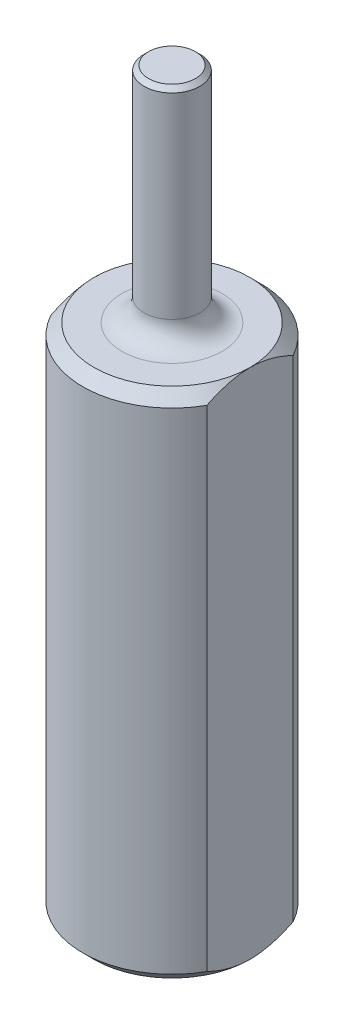
from build123d import *

# Parameters (mm, degrees)
HOLE_WIZARD_M3_1_D     = 2.5
HOLE_WIZARD_M3_1_DEPTH = 11.5
HOLE_WIZARD_M3_1_TIP   = 0.751075774
CHAMFER_1_SIZE         = 0.5
FILLET_1_R             = 1
SKETCH_4_W             = 0.5
SKETCH_4_H             = 23
CUT_EXTRUDE_1_DEPTH    = 5
CHAMFER_2_SIZE         = 0.2


with BuildPart() as part:
    # 草图1 → 旋转1 (revolve)
    with BuildSketch(Plane.XY, mode=Mode.PRIVATE) as revolve_1_sk:
        Polygon((1.25, 33), (1.25, 23), (4, 23), (4, 0), (0, 0), (0, 33), align=None)
    revolve(revolve_1_sk.sketch.rotate(Axis((0, -0.524377328, 0), (0, 1, 0)), 90), axis=Axis((0, -0.524377328, 0), (0, 1, 0)))

    # M3 螺纹孔1
    with Locations(Plane(origin=(0, 0, 0), x_dir=(-1, 0, 0), z_dir=(0, -1, 0))):
        with Locations((0, 0)):
            Hole(HOLE_WIZARD_M3_1_D / 2, depth=HOLE_WIZARD_M3_1_DEPTH)
            with Locations((0, 0, -(HOLE_WIZARD_M3_1_DEPTH + HOLE_WIZARD_M3_1_TIP / 2))):  # 118° drill point
                Cone(0, HOLE_WIZARD_M3_1_D / 2, HOLE_WIZARD_M3_1_TIP, mode=Mode.SUBTRACT)

    # 倒角1
    chamfer_1_edges = [part.edges().sort_by_distance(p)[0] for p in [
        (0, 0, 4),
        (0, 23, 4),
    ]]
    chamfer(chamfer_1_edges, length=CHAMFER_1_SIZE)

    # 圆角1
    fillet_1_edges = [part.edges().sort_by_distance(p)[0] for p in [
        (0, 23, 1.25),
    ]]
    fillet(fillet_1_edges, radius=FILLET_1_R)

    # 草图4 → 切除-拉伸1 (cut, symmetric)
    with BuildSketch(Plane.XY):
        with Locations((3.75, 11.5)):
            Rectangle(SKETCH_4_W, SKETCH_4_H)
        with Locations((-3.75, 11.5)):
            Rectangle(SKETCH_4_W, SKETCH_4_H)
    extrude(amount=CUT_EXTRUDE_1_DEPTH, both=True, mode=Mode.SUBTRACT)

    # 倒角2
    chamfer_2_edges = [part.edges().sort_by_distance(p)[0] for p in [
        (0, 33, 1.25),
    ]]
    chamfer(chamfer_2_edges, length=CHAMFER_2_SIZE)


solid = part.part
